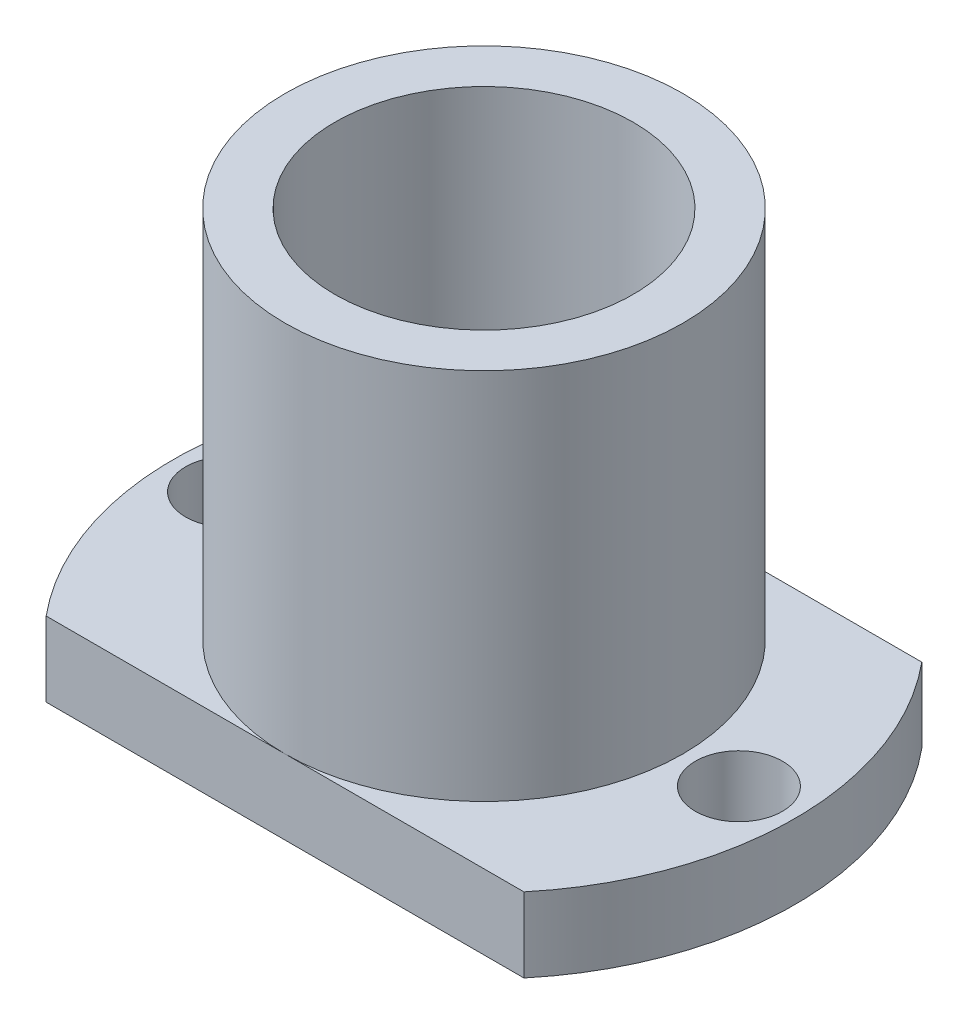
from build123d import *

# Parameters (mm, degrees)
SKETCH2_R          = 3.5
CUT_EXTRUDE1_DEPTH = 47.368092477
CUT_EXTRUDE2_DEPTH = 47.368092477


with BuildPart() as part:
    # Sketch1 → Revolve1 (revolve)
    with BuildSketch(Plane.XY, mode=Mode.PRIVATE) as revolve1_sk:
        Polygon((12, 36), (12, 0), (25, 0), (25, 6), (16, 6), (16, 36), align=None)
    revolve(revolve1_sk.sketch.rotate(Axis((0, 0, 0), (0, 1, 0)), 90), axis=Axis((0, 0, 0), (0, 1, 0)))

    # Sketch2 → Cut-Extrude1 (cut, through all)
    with BuildSketch(Plane(origin=(0, 6, 0), x_dir=(1, 0, 0), z_dir=(0, 1, 0))):
        with Locations(Location((-20.5, 0, 0), (0, 0, 270))):
            Circle(SKETCH2_R)
        with Locations(Location((0, 20.5, 0), (0, 0, 270))):
            Circle(SKETCH2_R)
        with Locations(Location((20.5, 0, 0), (0, 0, 270))):
            Circle(SKETCH2_R)
        with Locations(Location((0, -20.5, 0), (0, 0, 270))):
            Circle(SKETCH2_R)
    extrude(amount=-CUT_EXTRUDE1_DEPTH, mode=Mode.SUBTRACT)

    # Sketch3 → Cut-Extrude2 (cut, through all)
    with BuildSketch(Plane(origin=(0, 6, 0), x_dir=(1, 0, 0), z_dir=(0, 1, 0))):
        with BuildLine():
            Line((-19.209372712, 16), (19.209372712, 16))
            ThreePointArc((19.209372712, 16), (0, 25), (-19.209372712, 16))
        make_face()
        with BuildLine():
            Line((-19.209372712, -16), (19.209372712, -16))
            ThreePointArc((19.209372712, -16), (0, -25), (-19.209372712, -16))
        make_face()
    extrude(amount=-CUT_EXTRUDE2_DEPTH, mode=Mode.SUBTRACT)


solid = part.part
